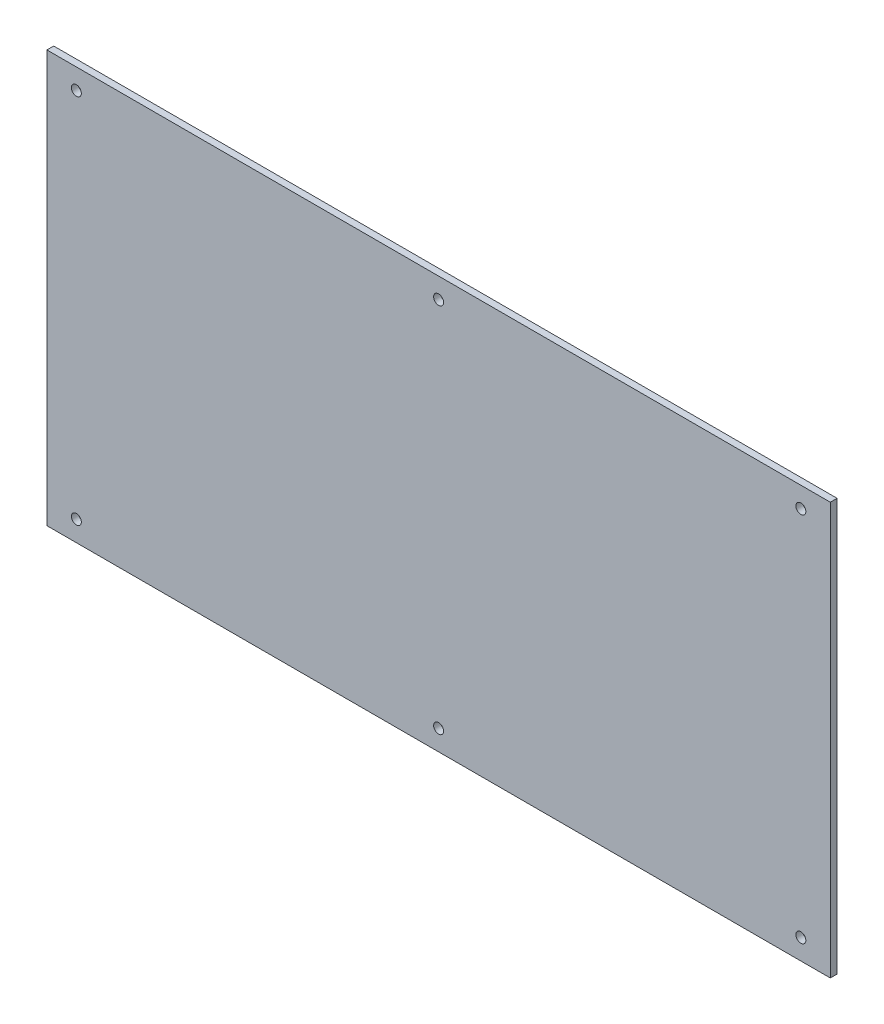
SolidWorks part; units mm, degrees
ref_plane "前视基准面" through (0, 0, 0) normal (0, 0, 1) x (1, 0, 0)
ref_plane "上视基准面" through (0, 0, 0) normal (0, 1, 0) x (1, 0, 0)
ref_plane "右视基准面" through (0, 0, 0) normal (1, 0, 0) x (0, 0, -1)
sketch "草图1" plane through (0, 0, 0) normal (0, 0, 1) x (1, 0, 0)
  line L1 (173, -91) -> (-173, -91)
  line L2 (173, -91) -> (173, 91)
  line L3 (173, 91) -> (-173, 91)
  line L4 (-173, -91) -> (-173, 91)
  line L5 (173, -91) -> (-173, 91) construction
  line L6 (173, 91) -> (-173, -91) construction
  point P0 (0, 0)
  dimension "D1" = 346
  dimension "D2" = 182
extrude "凸台-拉伸1" add sketch "草图1" along normal blind 3
sketch "草图2" plane through (0, 0, 0) normal (0, 0, -1) x (-1, 0, 0)
  line L4 (160, -82) -> (160, 82) construction
  line L5 (-160, 82) -> (-160, -82) construction
  line L8 (164, -82) -> (164, 82)
  line L9 (164, 82) -> (-164, 82)
  line L10 (-164, 82) -> (-164, -82)
  line L11 (-164, -82) -> (164, -82)
  line L12 (164, -82) -> (164, 82) construction
  line L13 (164, 82) -> (-164, 82) construction
  line L14 (-164, 82) -> (-164, -82) construction
  line L15 (-164, -82) -> (164, -82) construction
  circle A2 centre (0, 82) radius 2.2
  circle A4 centre (160, 82) radius 2.2
  circle A5 centre (0, -82) radius 2.2
  circle A6 centre (160, -82) radius 2.2
  circle A7 centre (-160, -82) radius 2.2
  circle A8 centre (-160, 82) radius 2.2
  dimension "D4" = 4.4
  dimension "D1" = 9
  dimension "D2" = 4
  dimension "D3" = 4
extrude "切除-拉伸1" cut sketch "草图2" against normal blind 10
